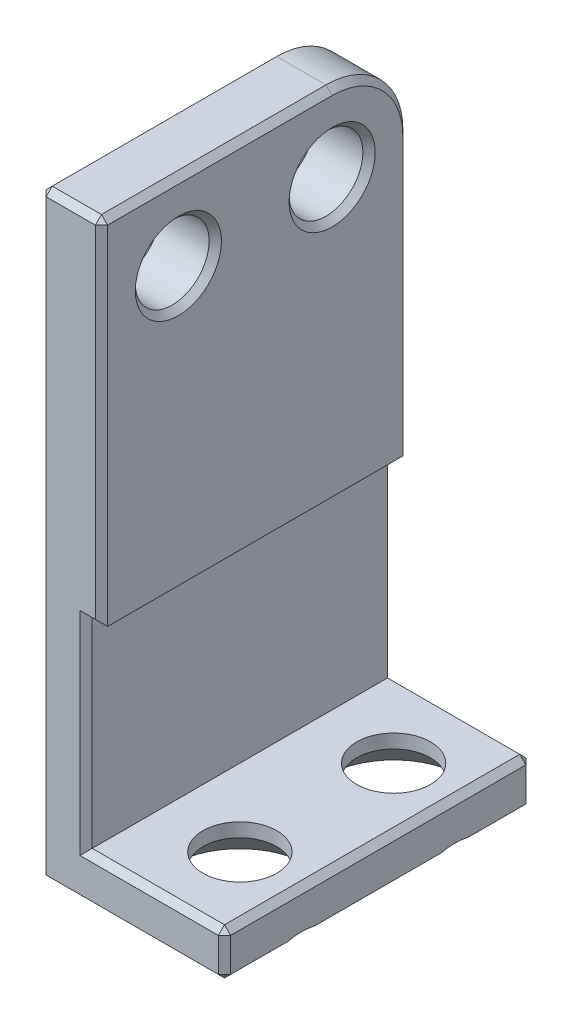
from build123d import *

# Parameters (mm, degrees)
SKETCH1_W                                    = 2
SKETCH1_H                                    = 10
BOSS_EXTRUDE1_DEPTH                          = 19.5
SKETCH2_R                                    = 1.2
CUT_EXTRUDE1_DEPTH                           = 20
SKETCH3_W                                    = 10
SKETCH3_H                                    = 1.5
BOSS_EXTRUDE2_DEPTH                          = 4
SKETCH4_W                                    = 10
SKETCH4_H                                    = 6.5
CUT_EXTRUDE2_DEPTH                           = 0.5
HOLE_SIZE_SLOTTED_COUNTERSUNK_WOOD_S_2_COUNT = 2
HOLE_SIZE_SLOTTED_COUNTERSUNK_WOOD_S_2_PITCH = 5
FILLET1_R                                    = 2.5
CHAMFER1_SIZE                                = 0.2


with BuildPart() as part:
    # Sketch1 → Boss-Extrude1 (new body)
    with BuildSketch(Plane(origin=(0, 0, 0), x_dir=(1, 0, 0), z_dir=(0, 1, 0))):
        with Locations((1, 5)):
            Rectangle(SKETCH1_W, SKETCH1_H)
    extrude(amount=BOSS_EXTRUDE1_DEPTH)

    # Sketch2 → Cut-Extrude1 (cut)
    with BuildSketch(Plane(origin=(2, 0, 0), x_dir=(0, 0, -1), z_dir=(1, 0, 0))):
        with Locations((2.5, 17)):
            Circle(SKETCH2_R)
        with Locations((7.5, 17)):
            Circle(SKETCH2_R)
    extrude(amount=-CUT_EXTRUDE1_DEPTH, mode=Mode.SUBTRACT)

    # Sketch3 → Boss-Extrude2 (add)
    with BuildSketch(Plane(origin=(2, 0, 0), x_dir=(0, 0, -1), z_dir=(1, 0, 0))):
        with Locations((5, 0.75)):
            Rectangle(SKETCH3_W, SKETCH3_H)
    extrude(amount=BOSS_EXTRUDE2_DEPTH)

    # Sketch4 → Cut-Extrude2 (cut)
    with BuildSketch(Plane(origin=(2, 0, 0), x_dir=(0, 0, -1), z_dir=(1, 0, 0))):
        with Locations((5, 4.75)):
            Rectangle(SKETCH4_W, SKETCH4_H)
    extrude(amount=-CUT_EXTRUDE2_DEPTH, mode=Mode.SUBTRACT)

    # Sketch6 → Hole size slotted countersunk wood screw type 0 (revolve, cut)
    with BuildSketch(Plane(origin=(4, 0, -2.5), x_dir=(0, 0, -1), z_dir=(1, 0, 0))):
        Polygon((0, 0), (0, 1.5), (1.2, 1.5), (1.2, 1.05), (2.25, 0), align=None)
    hole_size_slotted_countersunk_wood_screw = revolve(axis=Axis((4, -6.35, -2.5), (0, 1, 0)), mode=Mode.SUBTRACT)

    # Hole size slotted countersunk wood s 2: Hole size slotted countersunk wood screw type 0 ×2
    with Locations(*[(0, 0, -i * HOLE_SIZE_SLOTTED_COUNTERSUNK_WOOD_S_2_PITCH) for i in range(1, HOLE_SIZE_SLOTTED_COUNTERSUNK_WOOD_S_2_COUNT)]):
        add(hole_size_slotted_countersunk_wood_screw, mode=Mode.SUBTRACT)

    # Fillet1
    fillet1_edges = [part.edges().sort_by_distance(p)[0] for p in [
        (1, 19.5, -10),
    ]]
    fillet(fillet1_edges, radius=FILLET1_R)

    # Chamfer1
    chamfer1_edges = [part.edges().sort_by_distance(p)[0] for p in [
        (0, 17, -6.3),
        (0, 17, -1.3),
        (6, 0, -5),
        (2, 19.5, -3.75),
        (2, 18.767766953, -9.267766953),
        (3, 0, -10),
        (6, 0, -9.265388203),
        (6, 0.75, -10),
        (2, 12.5, -10),
        (1.75, 8, -10),
        (1.5, 4.75, -10),
        (3.75, 1.5, -10),
        (3.75, 1.5, 0),
        (1.5, 4.75, 0),
        (1.75, 8, 0),
        (2, 13.75, 0),
        (1, 19.5, 0),
        (0, 9.75, 0),
        (0, 19.5, -3.75),
        (0, 18.767766953, -9.267766953),
        (0, 8.5, -10),
        (0, 0, -5),
        (3, 0, 0),
        (6, 0, -0.734611797),
        (6, 0.75, 0),
        (6, 1.5, -5),
        (2, 17, -1.3),
        (2, 17, -6.3),
    ]]
    chamfer(chamfer1_edges, length=CHAMFER1_SIZE)


solid = part.part
